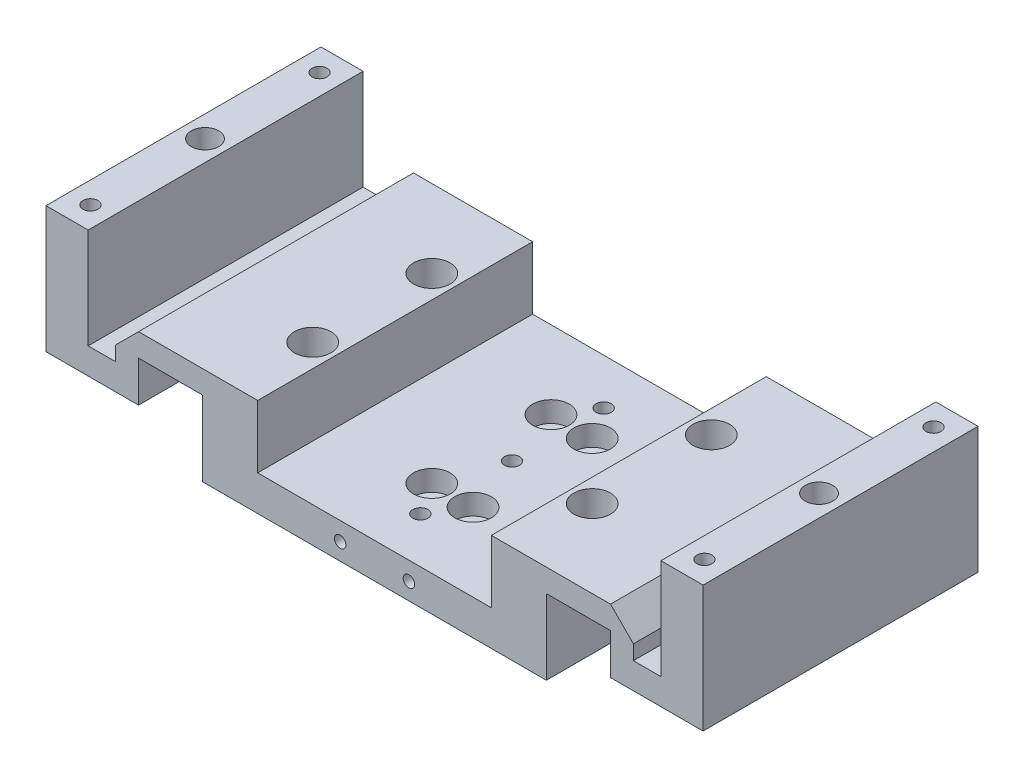
SolidWorks part; units mm, degrees
material "GY-D-143HT 型材"
ref_plane "前视基准面" through (0, 0, 0) normal (0, 0, 1) x (1, 0, 0)
ref_plane "上视基准面" through (0, 0, 0) normal (0, 1, 0) x (1, 0, 0)
ref_plane "右视基准面" through (0, 0, 0) normal (1, 0, 0) x (0, 0, -1)
sketch "草图1" plane through (0, 0, 0) normal (0, 0, 1) x (1, 0, 0)
  line L0 (0, 0) -> (0, 40.0158) construction
  line L1 (37.5, 0) -> (-37.5, 0)
  line L2 (-37.5, 0) -> (-37.5, 16.3882)
  line L3 (-37.5, 16.3882) -> (-51.5, 16.3882)
  line L4 (-51.5, 16.3882) -> (-51.5, 7.5)
  line L5 (-51.5, 7.5) -> (-71.7, 7.5)
  line L6 (-71.7, 7.5) -> (-71.7, 35.1)
  line L7 (-71.7, 35.1) -> (-62.5, 35.1)
  line L8 (-62.5, 35.1) -> (-62.5, 13.2)
  line L9 (-62.5, 13.2) -> (-56.5, 13.2)
  line L10 (-56.5, 13.2) -> (-56.5, 21.3882)
  line L11 (-56.5, 21.3882) -> (-25.5, 21.3882)
  line L12 (-25.5, 21.3882) -> (-25.5, 7.7)
  line L13 (-25.5, 7.7) -> (25.5, 7.7)
  line L14 (25.5, 21.3882) -> (25.5, 7.7)
  line L15 (56.5, 21.3882) -> (25.5, 21.3882)
  line L16 (56.5, 13.2) -> (56.5, 21.3882)
  line L17 (62.5, 13.2) -> (56.5, 13.2)
  line L18 (62.5, 35.1) -> (62.5, 13.2)
  line L19 (71.7, 35.1) -> (62.5, 35.1)
  line L20 (71.7, 7.5) -> (71.7, 35.1)
  line L21 (51.5, 7.5) -> (71.7, 7.5)
  line L22 (51.5, 16.3882) -> (51.5, 7.5)
  line L23 (37.5, 16.3882) -> (51.5, 16.3882)
  line L24 (37.5, 0) -> (37.5, 16.3882)
  point P17 (0, 7.7)
  dimension "D1" = 75
  dimension "D2" = 51
  dimension "D3" = 27.6
  dimension "D4" = 35.1
  dimension "D5" = 21.9
  dimension "D6" = 113
  dimension "D7" = 143.4
  dimension "D8" = 125
  dimension "D9" = 103
  dimension "D10" = 7.7
  dimension "D11" = 5
extrude "凸台-拉伸1" add sketch "草图1" along normal mid plane 60
chamfer "倒角1" distance 5 angle 45 2 edges at (56.5, 21.3882, 0) (-56.5, 21.3882, 0)
sketch "草图2" plane through (0, 0, 0) normal (0, -1, 0) x (1, 0, 0)
  line L0 (0, 30) -> (0, -30) construction
  line L1 (-37.5, 30) -> (37.5, 30) construction
  line L2 (-37.5, -30) -> (37.5, -30) construction
  line L3 (-37.5, 0) -> (37.5, 0) construction
  line L4 (-37.5, 30) -> (-37.5, -30) construction
  line L5 (37.5, 30) -> (37.5, -30) construction
  line L6 (-4.5, 13) -> (-30.5, 13) construction
  line L7 (4.5, 13) -> (30.5, 13) construction
  line L8 (4.5, -13) -> (30.5, -13) construction
  line L9 (-4.5, -13) -> (-30.5, -13) construction
  circle A0 centre (-4.5, 13) radius 2
  circle A1 centre (-30.5, 13) radius 2
  circle A2 centre (30.5, 13) radius 2
  circle A3 centre (4.5, 13) radius 2
  circle A4 centre (4.5, -13) radius 2
  circle A5 centre (30.5, -13) radius 2
  circle A6 centre (-30.5, -13) radius 2
  circle A7 centre (-4.5, -13) radius 2
  dimension "D2" = 4
  dimension "D3" = 9
  dimension "D4" = 26
  dimension "D1" = 26
extrude "切除-拉伸1" cut sketch "草图2" against normal through all
sketch "草图4" plane through (0, 21.3882, 0) normal (0, 1, 0) x (1, 0, 0)
  circle A0 centre (-30.5, 13) radius 3.5
  circle A1 centre (-30.5, -13) radius 3.5
  circle A2 centre (30.5, 13) radius 3.5
  circle A3 centre (30.5, -13) radius 3.5
  dimension "D1" = 7
extrude "切除-拉伸3" cut sketch "草图4" against normal blind 4.5
sketch "草图5" plane through (0, 7.7, 0) normal (0, 1, 0) x (1, 0, 0)
  circle A0 centre (-4.5, 13) radius 3.5
  circle A1 centre (4.5, 13) radius 3.5
  circle A2 centre (4.5, -13) radius 3.5
  circle A3 centre (-4.5, -13) radius 3.5
  dimension "D1" = 7
extrude "切除-拉伸4" cut sketch "草图5" against normal blind 4.5
hole_wizard "M4 螺纹孔1" positions "草图7" profile "草图6" tap size "M4" standard "GB"
sketch "草图7" plane through (0, 35.1, 0) normal (0, 1, 0) x (1, 0, 0)
  point P0 (-67, 25)
  dimension "D1" = 67
  dimension "D2" = 25
sketch "草图6" plane through (-67, 35.1, -25) normal (1, 0, 0) x (0, 0, 1)
  line L0 (0, 0) -> (0, 12.9914)
  line L1 (0, 12.9914) -> (1.65, 12)
  line L2 (1.65, 12) -> (1.65, 0)
  line L5 (1.65, 0) -> (0, 0)
  line L10 (0, 12.9914) -> (-1.65, 12) construction
  line L11 (0, -6.35) -> (0, 31.0958) construction
  dimension "螺纹孔钻头直径" = 3.3
  dimension "螺纹孔钻头深度" = 12
  dimension "导头角度" = 118
cosmetic thread "孔螺蚊线1" parameters "D1"=10, "D2"=4
mirror "镜向1" about plane through (0, 0, 0) normal (0, 0, 1) of "M4 螺纹孔1"
mirror "镜向2" about plane through (0, 0, 0) normal (1, 0, 0) of "M4 螺纹孔1", "镜向1"
hole_wizard "M3 螺纹孔5" positions "草图9" profile "草图8" tap size "M3" standard "GB"
sketch "草图9" plane through (0, 0, -30) normal (0, 0, -1) x (-1, 0, 0)
  line L0 (-33.5, 17) -> (-33.5, 11) construction
  line L2 (37.5, 0) -> (-37.5, 0) construction
  line L3 (-37.5, 0) -> (-37.5, 16.3882) construction
  point P0 (-33.5, 11)
  point P2 (-33.5, 17)
  dimension "D1" = 11
  dimension "D2" = 4
  dimension "D3" = 6
sketch "草图8" plane through (33.5, 11, -30) normal (1, 0, 0) x (0, 1, 0)
  line L0 (0, 0) -> (0, 9.2511)
  line L1 (0, 9.2511) -> (1.25, 8.5)
  line L2 (1.25, 8.5) -> (1.25, 0)
  line L5 (1.25, 0) -> (0, 0)
  line L10 (0, 9.2511) -> (-1.25, 8.5) construction
  line L11 (0, -6.35) -> (0, 14.638) construction
  dimension "螺纹孔钻头直径" = 2.5
  dimension "螺纹孔钻头深度" = 8.5
  dimension "导头角度" = 118
cosmetic thread "孔螺蚊线2" parameters "D1"=6, "D2"=3
cosmetic thread "孔螺蚊线3" parameters "D1"=6, "D2"=3
hole_wizard "M3 螺纹孔4" positions "草图11" profile "草图10" tap size "M3" standard "GB"
sketch "草图11" plane through (0, 0, 30) normal (0, 0, 1) x (1, 0, 0)
  line L0 (-33.5, 13) -> (-33.5, 19) construction
  line L2 (-37.5, 0) -> (37.5, 0) construction
  line L3 (-37.5, 16.3882) -> (-37.5, 0) construction
  point P0 (-33.5, 13)
  point P2 (-33.5, 19)
  dimension "D1" = 13
  dimension "D2" = 6
  dimension "D3" = 4
sketch "草图10" plane through (-33.5, 13, 30) normal (1, 0, 0) x (0, -1, 0)
  line L0 (0, 0) -> (0, 9.2511)
  line L1 (0, 9.2511) -> (1.25, 8.5)
  line L2 (1.25, 8.5) -> (1.25, 0)
  line L5 (1.25, 0) -> (0, 0)
  line L10 (0, 9.2511) -> (-1.25, 8.5) construction
  line L11 (0, -6.35) -> (0, 16.8953) construction
  dimension "螺纹孔钻头直径" = 2.5
  dimension "螺纹孔钻头深度" = 8.5
  dimension "导头角度" = 118
cosmetic thread "孔螺蚊线4" [suppressed] parameters "D1"=6, "D2"=3
cosmetic thread "孔螺蚊线5" [suppressed] parameters "D1"=6, "D2"=3
hole_wizard "M4 螺纹孔2" positions "草图13" profile "草图12" tap size "M4" standard "GB" end condition up to next
sketch "草图13" plane through (0, 0, 0) normal (0, -1, 0) x (-1, 0, 0)
  line L2 (25.5, -30) -> (25.5, 30) construction
  line L3 (-25.5, 30) -> (25.5, 30) construction
  point P0 (0, 20)
  dimension "D1" = 25.5
  dimension "D3" = 10
sketch "草图12" plane through (0, 0, -20) normal (1, 0, 0) x (0, 0, -1)
  line L0 (0, 0) -> (0, 7.701)
  line L1 (0, 7.701) -> (1.65, 7.701)
  line L2 (1.65, 7.701) -> (1.65, 0)
  line L5 (1.65, 0) -> (0, 0)
  line L11 (0, -6.35) -> (0, 107.95) construction
  dimension "通孔螺纹孔钻头直径" = 3.3
  dimension "通孔螺纹孔钻头深度" = 7.701
cosmetic thread "孔螺蚊线6" parameters "D2"=4
hole_wizard "M3 螺纹孔3" positions "草图15" profile "草图14" tap size "M3" standard "GB"
sketch "草图15" plane through (0, 0, 30) normal (0, 0, 1) x (1, 0, 0)
  line L0 (25.5, 7.7) -> (-25.5, 7.7) construction
  point P0 (-7.5, 3.7)
  dimension "D1" = 4
  dimension "D2" = 7.5
sketch "草图14" plane through (-7.5, 3.7, 30) normal (1, 0, 0) x (0, -1, 0)
  line L0 (0, 0) -> (0, 11.7511)
  line L1 (0, 11.7511) -> (1.25, 11)
  line L2 (1.25, 11) -> (1.25, 0)
  line L5 (1.25, 0) -> (0, 0)
  line L10 (0, 11.7511) -> (-1.25, 11) construction
  line L11 (0, -6.35) -> (0, 107.95) construction
  dimension "螺纹孔钻头直径" = 2.5
  dimension "螺纹孔钻头深度" = 11
  dimension "导头角度" = 118
cosmetic thread "孔螺蚊线7" parameters "D1"=10, "D2"=3
mirror "镜向4" about plane through (0, 0, 0) normal (1, 0, 0) of "M3 螺纹孔3"
mirror "镜向5" about plane through (0, 0, 0) normal (0, 0, 1) of "M3 螺纹孔3", "镜向4"
hole_wizard "打孔尺寸(%根据)开槽圆柱头螺钉的类型2" positions "草图17" profile "草图16" counterbore size "M4" standard "GB" end condition through all
sketch "草图17" plane through (0, 21.3882, 0) normal (0, 1, 0) x (1, 0, 0)
  point P0 (-30.5, 13)
  point P3 (-30.5, -13)
  point P6 (30.5, 13)
  point P9 (30.5, -13)
sketch "草图16" plane through (-30.5, 21.3882, -13) normal (1, 0, 0) x (0, 0, 1)
  line L0 (0, 0) -> (0, 21.3882)
  line L1 (0, 21.3882) -> (2.25, 21.3882)
  line L3 (2.25, 21.3882) -> (2.25, 6)
  line L4 (2.25, 6) -> (4, 6)
  line L5 (4, 6) -> (4, 0)
  line L7 (4, 0) -> (0, 0)
  line L11 (0, -6.35) -> (0, 107.95) construction
  dimension "通孔孔直径" = 4.5
  dimension "通孔孔深度" = 21.3882
  dimension "柱形沉头孔直径" = 8
  dimension "柱形沉头孔深度" = 6
hole_wizard "打孔尺寸(%根据)开槽圆柱头螺钉的类型2" positions "草图19" profile "草图18" counterbore size "M4" standard "GB" end condition through all
sketch "草图19" plane through (0, 7.7, 0) normal (0, 1, 0) x (1, 0, 0)
  point P0 (-4.5, 13)
  point P3 (4.5, 13)
  point P6 (-4.5, -13)
  point P9 (4.5, -13)
sketch "草图18" plane through (-4.5, 7.7, -13) normal (1, 0, 0) x (0, 0, 1)
  line L0 (0, 0) -> (0, 7.7)
  line L1 (0, 7.7) -> (2.25, 7.7)
  line L3 (2.25, 7.7) -> (2.25, 4.5)
  line L4 (2.25, 4.5) -> (4, 4.5)
  line L5 (4, 4.5) -> (4, 0)
  line L7 (4, 0) -> (0, 0)
  line L11 (0, -6.35) -> (0, 107.95) construction
  dimension "通孔孔直径" = 4.5
  dimension "通孔孔深度" = 7.7
  dimension "柱形沉头孔直径" = 8
  dimension "柱形沉头孔深度" = 4.5
pattern_linear "阵列(线性)1" count 3 spacing 20 along (0, 0, 1) of "M4 螺纹孔2"
hole_wizard "大小mm 暗销孔1" positions "草图20" profile "草图22" hole size "Ø6.0" standard "GB"
sketch "草图20" plane through (0, 35.1, 0) normal (0, 1, 0) x (1, 0, 0)
  line L0 (67, 25) -> (67, -25) construction
  point P0 (67, 0)
sketch "草图22" plane through (67, 35.1, 0) normal (1, 0, 0) x (0, 0, 1)
  line L0 (0, 0) -> (0, 16.8026)
  line L1 (0, 16.8026) -> (3, 15)
  line L2 (3, 15) -> (3, 0)
  line L5 (3, 0) -> (0, 0)
  line L10 (0, 16.8026) -> (-3, 15) construction
  line L11 (0, -6.35) -> (0, 107.95) construction
  dimension "孔直径" = 6
  dimension "孔深度" = 15
  dimension "导头角度" = 118
mirror "镜向6" about plane through (0, 0, 0) normal (1, 0, 0) of "大小mm 暗销孔1"
